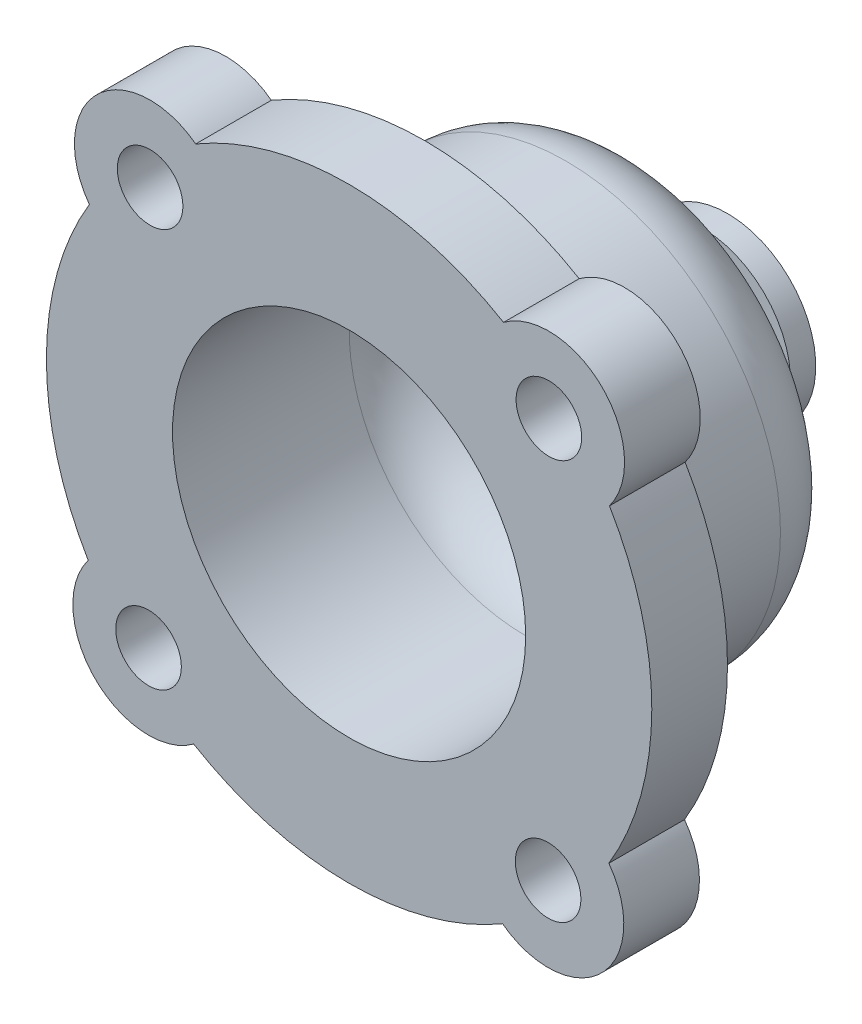
SolidWorks part; units mm, degrees
ref_plane "Front Plane" through (0, 0, 0) normal (0, 0, 1) x (1, 0, 0)
ref_plane "Top Plane" through (0, 0, 0) normal (0, 1, 0) x (1, 0, 0)
ref_plane "Right Plane" through (0, 0, 0) normal (1, 0, 0) x (0, 0, -1)
sketch "Sketch1" plane through (0, 0, 0) normal (0, 0, 1) x (1, 0, 0)
  line L0 (0, 60) -> (0, -60) construction
  line L1 (39.598, 39.598) -> (0, 0) construction
  line L2 (0, 0) -> (-39.4456, 39.7497) construction
  line L3 (0, 0) -> (39.4456, -39.7497) construction
  line L4 (0, 0) -> (-39.7497, -39.4456) construction
  circle A0 centre (0, 0) radius 56 construction
  arc A1 (30.6082, 51.6056) -> (-30.4098, 51.7228) centre (0, 0) ccw
  circle A2 centre (39.598, 39.598) radius 6.5
  arc A3 (51.6056, 30.6082) -> (30.6082, 51.6056) centre (39.598, 39.598) ccw
  arc A4 (-30.4098, 51.7228) -> (-51.4877, 30.8061) centre (-39.4456, 39.7497) ccw
  circle A5 centre (-39.4456, 39.7497) radius 6.5
  arc A6 (-51.4877, 30.8061) -> (-51.7228, -30.4098) centre (0, 0) ccw
  arc A7 (-51.7228, -30.4098) -> (-30.8061, -51.4877) centre (-39.7497, -39.4456) ccw
  arc A8 (30.4098, -51.7228) -> (51.4877, -30.8061) centre (39.4456, -39.7497) ccw
  circle A9 centre (-39.7497, -39.4456) radius 6.5
  circle A10 centre (39.4456, -39.7497) radius 6.5
  arc A11 (-30.8061, -51.4877) -> (30.4098, -51.7228) centre (0, 0) ccw
  arc A12 (51.4877, -30.8061) -> (51.6056, 30.6082) centre (0, 0) ccw
  dimension "D1" = 112
  dimension "D2" = 120
  dimension "D4" = 30
  dimension "D5" = 13
  dimension "D7" = 30
  dimension "D8" = 13
  dimension "D11" = 13
  dimension "D3" = 45
  dimension "D6" = 44.78
  dimension "D9" = 45.22
  dimension "D10" = 44.78
extrude "Boss-Extrude1" add sketch "Sketch1" along normal blind 15
sketch "Sketch2" plane through (0, 0, 15) normal (0, 0, 1) x (1, 0, 0)
  circle A0 centre (-39.4456, 39.7497) radius 13
  circle A1 centre (39.598, 39.598) radius 13
  circle A2 centre (39.4456, -39.7497) radius 13
  circle A3 centre (-39.7497, -39.4456) radius 13
  dimension "D1" = 26
extrude "Cut-Extrude1" cut sketch "Sketch2" against normal blind 2 from offset 13 offset against normal yes
sketch "Sketch3" plane through (0, 0, 0) normal (0, 1, 0) x (1, 0, 0)
  line L0 (-42.5, 0) -> (-42.5, 43)
  line L1 (-30.4098, 0) -> (-54.4456, 0) construction
  line L2 (-42.5, 43) -> (-17.5, 43)
  line L3 (-17.5, 43) -> (-17.5, 50)
  line L4 (-17.5, 55) -> (-15, 55)
  line L5 (-15, 55) -> (-15, 50)
  line L6 (-15, 50) -> (-17.5, 50)
  line L7 (-17.5, 55) -> (-17.5, 60)
  line L8 (-17.5, 60) -> (0, 60)
  line L9 (-54.4456, -15) -> (-30.4098, -15) construction
  line L10 (-30.4098, -15) -> (30.6082, -15) construction
  line L11 (0, 60) -> (0, 0) construction
  line L12 (-42.5, 0) -> (0, 0)
  line L13 (0, 0) -> (0, 60)
  dimension "D1" = 42.5
  dimension "D2" = 43
  dimension "D3" = 17.5
  dimension "D4" = 15
  dimension "D5" = 65
  dimension "D6" = 5
  dimension "D7" = 75
revolve "Revolve1" add sketch "Sketch3" angle 360 about L11
fillet "Fillet1" radius 15 1 edges at (-42.5, 0, -43)
sketch "Sketch4" plane through (0, 0, -43) normal (0, 0, -1) x (-1, 0, 0)
  circle A0 centre (0, 0) radius 27.5
  dimension "D1" = 55
extrude "Boss-Extrude2" add sketch "Sketch4" along normal blind 2
sketch "Sketch5" plane through (0, 0, -60) normal (0, 0, -1) x (-1, 0, 0)
  circle A0 centre (0, 0) radius 7.25
  dimension "D1" = 14.5
extrude "Cut-Extrude2" cut sketch "Sketch5" against normal blind 30
sketch "Sketch6" plane through (0, 0, 15) normal (0, 0, 1) x (1, 0, 0)
  circle A0 centre (0, 0) radius 35
  dimension "D1" = 70
extrude "Cut-Extrude3" cut sketch "Sketch6" against normal blind 50
fillet "Fillet2" radius 15 1 edges at (35, 0, -35)
